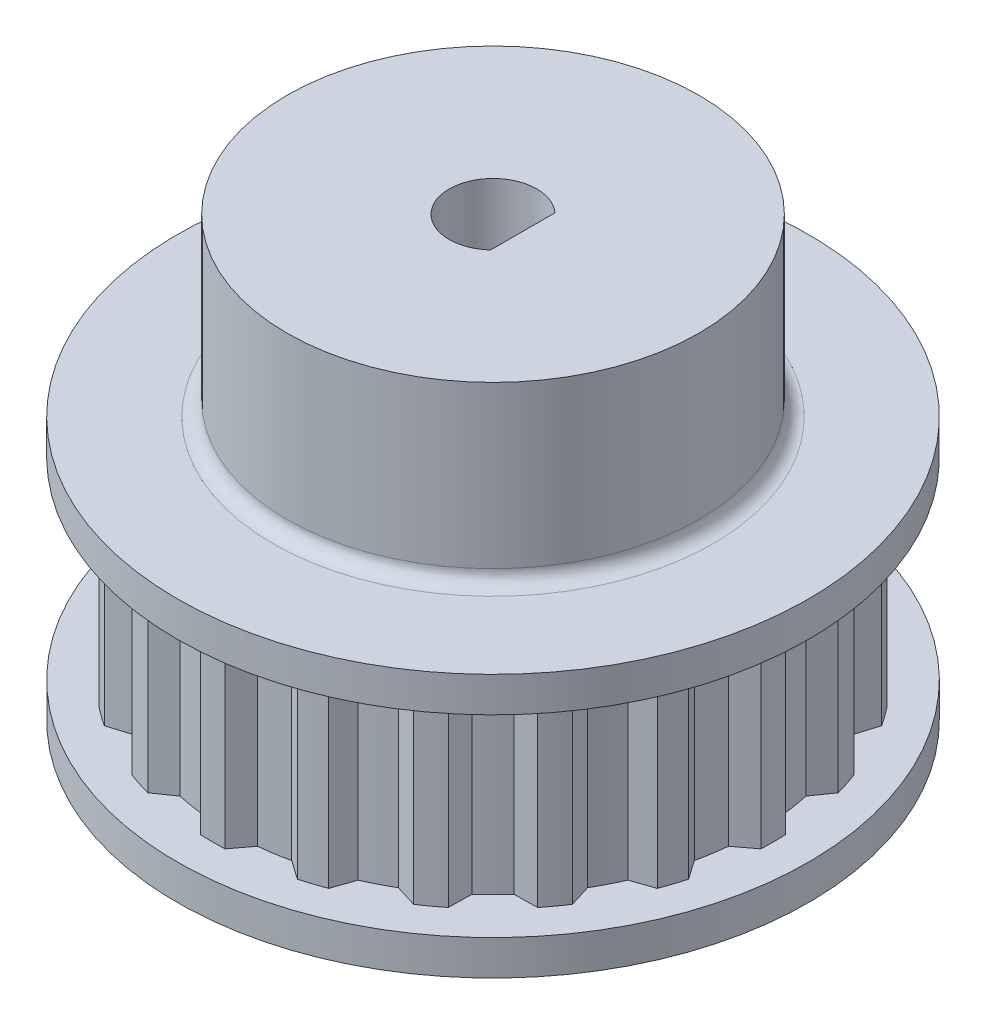
SolidWorks part; units mm, degrees
ref_plane "Front Plane" through (0, 0, 0) normal (0, 0, 1) x (1, 0, 0)
ref_plane "Top Plane" through (0, 0, 0) normal (0, 1, 0) x (1, 0, 0)
ref_plane "Right Plane" through (0, 0, 0) normal (1, 0, 0) x (0, 0, -1)
sketch "Sketch1" plane through (0, 0, 0) normal (0, 1, 0) x (1, 0, 0)
  circle A0 centre (0, 0) radius 16
  dimension "D1" = 32
extrude "Boss-Extrude1" add sketch "Sketch1" along normal blind 11
sketch "Sketch2" plane through (0, 11, 0) normal (0, 1, 0) x (1, 0, 0)
  line L0 (0, 21.2272) -> (0, -27.4763) construction
  line L1 (-1.5, 14.9329) -> (-0.7089, 15.9843)
  line L2 (1.5, 14.9329) -> (0.7089, 15.9843)
  line L3 (3.1879, 14.6656) -> (4.2652, 15.421)
  line L4 (6.0411, 13.7385) -> (5.6137, 14.9829)
  line L5 (7.5638, 12.9627) -> (8.8218, 13.3483)
  line L6 (9.9909, 11.1993) -> (9.9689, 12.5149)
  line L7 (11.1993, 9.9909) -> (12.5149, 9.9689)
  line L8 (12.9627, 7.5638) -> (13.3483, 8.8218)
  line L9 (13.7385, 6.0411) -> (14.9829, 5.6137)
  line L10 (14.6656, 3.1879) -> (15.421, 4.2652)
  line L11 (14.9329, 1.5) -> (15.9843, 0.7089)
  line L12 (14.9329, -1.5) -> (15.9843, -0.7089)
  line L13 (14.6656, -3.1879) -> (15.421, -4.2652)
  line L14 (13.7385, -6.0411) -> (14.9829, -5.6137)
  line L15 (12.9627, -7.5638) -> (13.3483, -8.8218)
  line L16 (11.1993, -9.9909) -> (12.5149, -9.9689)
  line L17 (9.9909, -11.1993) -> (9.9689, -12.5149)
  line L18 (7.5638, -12.9627) -> (8.8218, -13.3483)
  line L19 (6.0411, -13.7385) -> (5.6137, -14.9829)
  line L20 (3.1879, -14.6656) -> (4.2652, -15.421)
  line L21 (1.5, -14.9329) -> (0.7089, -15.9843)
  line L22 (-1.5, -14.9329) -> (-0.7089, -15.9843)
  line L23 (-3.1879, -14.6656) -> (-4.2652, -15.421)
  line L24 (-6.0411, -13.7385) -> (-5.6137, -14.9829)
  line L25 (-7.5638, -12.9627) -> (-8.8218, -13.3483)
  line L26 (-9.9909, -11.1993) -> (-9.9689, -12.5149)
  line L27 (-11.1993, -9.9909) -> (-12.5149, -9.9689)
  line L28 (-12.9627, -7.5638) -> (-13.3483, -8.8218)
  line L29 (-13.7385, -6.0411) -> (-14.9829, -5.6137)
  line L30 (-14.6656, -3.1879) -> (-15.421, -4.2652)
  line L31 (-14.9329, -1.5) -> (-15.9843, -0.7089)
  line L32 (-14.9329, 1.5) -> (-15.9843, 0.7089)
  line L33 (-14.6656, 3.1879) -> (-15.421, 4.2652)
  line L34 (-13.7385, 6.0411) -> (-14.9829, 5.6137)
  line L35 (-12.9627, 7.5638) -> (-13.3483, 8.8218)
  line L36 (-11.1993, 9.9909) -> (-12.5149, 9.9689)
  line L37 (-9.9909, 11.1993) -> (-9.9689, 12.5149)
  line L38 (-7.5638, 12.9627) -> (-8.8218, 13.3483)
  line L39 (-6.0411, 13.7385) -> (-5.6137, 14.9829)
  line L40 (-3.1879, 14.6656) -> (-4.2652, 15.421)
  arc A0 (-1.5, 14.9329) -> (-3.1879, 14.6656) centre (0, 0) ccw
  circle A1 centre (0, 0) radius 16 construction
  arc A3 (-1.5, 14.9329) -> (-3.1879, 14.6656) centre (0, 0) ccw
  arc A4 (5.6137, 14.9829) -> (4.2652, 15.421) centre (0, 0) ccw
  arc A5 (-1.5, 14.9329) -> (-3.1879, 14.6656) centre (0, 0) ccw
  arc A6 (9.9689, 12.5149) -> (8.8218, 13.3483) centre (0, 0) ccw
  arc A7 (-1.5, 14.9329) -> (-3.1879, 14.6656) centre (0, 0) ccw
  arc A8 (13.3483, 8.8218) -> (12.5149, 9.9689) centre (0, 0) ccw
  arc A9 (-1.5, 14.9329) -> (-3.1879, 14.6656) centre (0, 0) ccw
  arc A10 (15.9843, 0.7089) -> (15.421, 4.2652) centre (0, 0) ccw
  arc A11 (-1.5, 14.9329) -> (-3.1879, 14.6656) centre (0, 0) ccw
  arc A12 (15.421, -4.2652) -> (15.9843, -0.7089) centre (0, 0) ccw
  arc A13 (-1.5, 14.9329) -> (-3.1879, 14.6656) centre (0, 0) ccw
  arc A14 (13.3483, -8.8218) -> (14.9829, -5.6137) centre (0, 0) ccw
  arc A15 (-1.5, 14.9329) -> (-3.1879, 14.6656) centre (0, 0) ccw
  arc A16 (9.9689, -12.5149) -> (12.5149, -9.9689) centre (0, 0) ccw
  arc A17 (-1.5, 14.9329) -> (-3.1879, 14.6656) centre (0, 0) ccw
  arc A18 (5.6137, -14.9829) -> (8.8218, -13.3483) centre (0, 0) ccw
  arc A19 (-1.5, 14.9329) -> (-3.1879, 14.6656) centre (0, 0) ccw
  arc A20 (0.7089, -15.9843) -> (4.2652, -15.421) centre (0, 0) ccw
  arc A21 (-1.5, 14.9329) -> (-3.1879, 14.6656) centre (0, 0) ccw
  arc A22 (-4.2652, -15.421) -> (-0.7089, -15.9843) centre (0, 0) ccw
  arc A23 (-1.5, 14.9329) -> (-3.1879, 14.6656) centre (0, 0) ccw
  arc A24 (-8.8218, -13.3483) -> (-5.6137, -14.9829) centre (0, 0) ccw
  arc A25 (-1.5, 14.9329) -> (-3.1879, 14.6656) centre (0, 0) ccw
  arc A26 (-12.5149, -9.9689) -> (-9.9689, -12.5149) centre (0, 0) ccw
  arc A27 (-1.5, 14.9329) -> (-3.1879, 14.6656) centre (0, 0) ccw
  arc A28 (-14.9829, -5.6137) -> (-13.3483, -8.8218) centre (0, 0) ccw
  arc A29 (-1.5, 14.9329) -> (-3.1879, 14.6656) centre (0, 0) ccw
  arc A30 (-15.9843, -0.7089) -> (-15.421, -4.2652) centre (0, 0) ccw
  arc A31 (-1.5, 14.9329) -> (-3.1879, 14.6656) centre (0, 0) ccw
  arc A32 (-15.421, 4.2652) -> (-15.9843, 0.7089) centre (0, 0) ccw
  arc A33 (-1.5, 14.9329) -> (-3.1879, 14.6656) centre (0, 0) ccw
  arc A34 (-13.3483, 8.8218) -> (-14.9829, 5.6137) centre (0, 0) ccw
  arc A35 (-1.5, 14.9329) -> (-3.1879, 14.6656) centre (0, 0) ccw
  arc A36 (-9.9689, 12.5149) -> (-12.5149, 9.9689) centre (0, 0) ccw
  arc A37 (-1.5, 14.9329) -> (-3.1879, 14.6656) centre (0, 0) ccw
  arc A38 (-5.6137, 14.9829) -> (-8.8218, 13.3483) centre (0, 0) ccw
  arc A39 (-1.5, 14.9329) -> (-3.1879, 14.6656) centre (0, 0) ccw
  arc A40 (-0.7089, 15.9843) -> (-4.2652, 15.421) centre (0, 0) ccw
  arc A41 (3.1879, 14.6656) -> (1.5, 14.9329) centre (0, 0) ccw
  arc A42 (3.1879, 14.6656) -> (1.5, 14.9329) centre (0, 0) ccw
  arc A43 (3.1879, 14.6656) -> (1.5, 14.9329) centre (0, 0) ccw
  arc A44 (3.1879, 14.6656) -> (1.5, 14.9329) centre (0, 0) ccw
  arc A45 (3.1879, 14.6656) -> (1.5, 14.9329) centre (0, 0) ccw
  arc A46 (3.1879, 14.6656) -> (1.5, 14.9329) centre (0, 0) ccw
  arc A47 (3.1879, 14.6656) -> (1.5, 14.9329) centre (0, 0) ccw
  arc A48 (3.1879, 14.6656) -> (1.5, 14.9329) centre (0, 0) ccw
  arc A49 (3.1879, 14.6656) -> (1.5, 14.9329) centre (0, 0) ccw
  arc A50 (3.1879, 14.6656) -> (1.5, 14.9329) centre (0, 0) ccw
  arc A51 (3.1879, 14.6656) -> (1.5, 14.9329) centre (0, 0) ccw
  arc A52 (3.1879, 14.6656) -> (1.5, 14.9329) centre (0, 0) ccw
  arc A53 (3.1879, 14.6656) -> (1.5, 14.9329) centre (0, 0) ccw
  arc A54 (3.1879, 14.6656) -> (1.5, 14.9329) centre (0, 0) ccw
  arc A55 (3.1879, 14.6656) -> (1.5, 14.9329) centre (0, 0) ccw
  arc A56 (3.1879, 14.6656) -> (1.5, 14.9329) centre (0, 0) ccw
  arc A57 (3.1879, 14.6656) -> (1.5, 14.9329) centre (0, 0) ccw
  arc A58 (3.1879, 14.6656) -> (1.5, 14.9329) centre (0, 0) ccw
  arc A59 (3.1879, 14.6656) -> (1.5, 14.9329) centre (0, 0) ccw
  arc A60 (3.1879, 14.6656) -> (1.5, 14.9329) centre (0, 0) ccw
  arc A61 (7.5638, 12.9627) -> (6.0411, 13.7385) centre (0, 0) ccw
  arc A62 (7.5638, 12.9627) -> (6.0411, 13.7385) centre (0, 0) ccw
  arc A63 (7.5638, 12.9627) -> (6.0411, 13.7385) centre (0, 0) ccw
  arc A64 (7.5638, 12.9627) -> (6.0411, 13.7385) centre (0, 0) ccw
  arc A65 (7.5638, 12.9627) -> (6.0411, 13.7385) centre (0, 0) ccw
  arc A66 (7.5638, 12.9627) -> (6.0411, 13.7385) centre (0, 0) ccw
  arc A67 (7.5638, 12.9627) -> (6.0411, 13.7385) centre (0, 0) ccw
  arc A68 (7.5638, 12.9627) -> (6.0411, 13.7385) centre (0, 0) ccw
  arc A69 (7.5638, 12.9627) -> (6.0411, 13.7385) centre (0, 0) ccw
  arc A70 (7.5638, 12.9627) -> (6.0411, 13.7385) centre (0, 0) ccw
  arc A71 (7.5638, 12.9627) -> (6.0411, 13.7385) centre (0, 0) ccw
  arc A72 (7.5638, 12.9627) -> (6.0411, 13.7385) centre (0, 0) ccw
  arc A73 (7.5638, 12.9627) -> (6.0411, 13.7385) centre (0, 0) ccw
  arc A74 (7.5638, 12.9627) -> (6.0411, 13.7385) centre (0, 0) ccw
  arc A75 (7.5638, 12.9627) -> (6.0411, 13.7385) centre (0, 0) ccw
  arc A76 (7.5638, 12.9627) -> (6.0411, 13.7385) centre (0, 0) ccw
  arc A77 (7.5638, 12.9627) -> (6.0411, 13.7385) centre (0, 0) ccw
  arc A78 (7.5638, 12.9627) -> (6.0411, 13.7385) centre (0, 0) ccw
  arc A79 (7.5638, 12.9627) -> (6.0411, 13.7385) centre (0, 0) ccw
  arc A80 (7.5638, 12.9627) -> (6.0411, 13.7385) centre (0, 0) ccw
  arc A81 (11.1993, 9.9909) -> (9.9909, 11.1993) centre (0, 0) ccw
  arc A82 (11.1993, 9.9909) -> (9.9909, 11.1993) centre (0, 0) ccw
  arc A83 (11.1993, 9.9909) -> (9.9909, 11.1993) centre (0, 0) ccw
  arc A84 (11.1993, 9.9909) -> (9.9909, 11.1993) centre (0, 0) ccw
  arc A85 (11.1993, 9.9909) -> (9.9909, 11.1993) centre (0, 0) ccw
  arc A86 (11.1993, 9.9909) -> (9.9909, 11.1993) centre (0, 0) ccw
  arc A87 (11.1993, 9.9909) -> (9.9909, 11.1993) centre (0, 0) ccw
  arc A88 (11.1993, 9.9909) -> (9.9909, 11.1993) centre (0, 0) ccw
  arc A89 (11.1993, 9.9909) -> (9.9909, 11.1993) centre (0, 0) ccw
  arc A90 (11.1993, 9.9909) -> (9.9909, 11.1993) centre (0, 0) ccw
  arc A91 (11.1993, 9.9909) -> (9.9909, 11.1993) centre (0, 0) ccw
  arc A92 (11.1993, 9.9909) -> (9.9909, 11.1993) centre (0, 0) ccw
  arc A93 (11.1993, 9.9909) -> (9.9909, 11.1993) centre (0, 0) ccw
  arc A94 (11.1993, 9.9909) -> (9.9909, 11.1993) centre (0, 0) ccw
  arc A95 (11.1993, 9.9909) -> (9.9909, 11.1993) centre (0, 0) ccw
  arc A96 (11.1993, 9.9909) -> (9.9909, 11.1993) centre (0, 0) ccw
  arc A97 (11.1993, 9.9909) -> (9.9909, 11.1993) centre (0, 0) ccw
  arc A98 (11.1993, 9.9909) -> (9.9909, 11.1993) centre (0, 0) ccw
  arc A99 (11.1993, 9.9909) -> (9.9909, 11.1993) centre (0, 0) ccw
  arc A100 (11.1993, 9.9909) -> (9.9909, 11.1993) centre (0, 0) ccw
  arc A101 (13.7385, 6.0411) -> (12.9627, 7.5638) centre (0, 0) ccw
  arc A102 (13.7385, 6.0411) -> (12.9627, 7.5638) centre (0, 0) ccw
  arc A103 (13.7385, 6.0411) -> (12.9627, 7.5638) centre (0, 0) ccw
  arc A104 (13.7385, 6.0411) -> (12.9627, 7.5638) centre (0, 0) ccw
  arc A105 (13.7385, 6.0411) -> (12.9627, 7.5638) centre (0, 0) ccw
  arc A106 (13.7385, 6.0411) -> (12.9627, 7.5638) centre (0, 0) ccw
  arc A107 (13.7385, 6.0411) -> (12.9627, 7.5638) centre (0, 0) ccw
  arc A108 (13.7385, 6.0411) -> (12.9627, 7.5638) centre (0, 0) ccw
  arc A109 (13.7385, 6.0411) -> (12.9627, 7.5638) centre (0, 0) ccw
  arc A110 (13.7385, 6.0411) -> (12.9627, 7.5638) centre (0, 0) ccw
  arc A111 (13.7385, 6.0411) -> (12.9627, 7.5638) centre (0, 0) ccw
  arc A112 (13.7385, 6.0411) -> (12.9627, 7.5638) centre (0, 0) ccw
  arc A113 (13.7385, 6.0411) -> (12.9627, 7.5638) centre (0, 0) ccw
  arc A114 (13.7385, 6.0411) -> (12.9627, 7.5638) centre (0, 0) ccw
  arc A115 (13.7385, 6.0411) -> (12.9627, 7.5638) centre (0, 0) ccw
  arc A116 (13.7385, 6.0411) -> (12.9627, 7.5638) centre (0, 0) ccw
  arc A117 (13.7385, 6.0411) -> (12.9627, 7.5638) centre (0, 0) ccw
  arc A118 (13.7385, 6.0411) -> (12.9627, 7.5638) centre (0, 0) ccw
  arc A119 (13.7385, 6.0411) -> (12.9627, 7.5638) centre (0, 0) ccw
  arc A120 (13.7385, 6.0411) -> (12.9627, 7.5638) centre (0, 0) ccw
  arc A121 (14.9329, 1.5) -> (14.6656, 3.1879) centre (0, 0) ccw
  arc A122 (14.9329, 1.5) -> (14.6656, 3.1879) centre (0, 0) ccw
  arc A123 (14.9329, 1.5) -> (14.6656, 3.1879) centre (0, 0) ccw
  arc A124 (14.9329, 1.5) -> (14.6656, 3.1879) centre (0, 0) ccw
  arc A125 (14.9329, 1.5) -> (14.6656, 3.1879) centre (0, 0) ccw
  arc A126 (14.9329, 1.5) -> (14.6656, 3.1879) centre (0, 0) ccw
  arc A127 (14.9329, 1.5) -> (14.6656, 3.1879) centre (0, 0) ccw
  arc A128 (14.9329, 1.5) -> (14.6656, 3.1879) centre (0, 0) ccw
  arc A129 (14.9329, 1.5) -> (14.6656, 3.1879) centre (0, 0) ccw
  arc A130 (14.9329, 1.5) -> (14.6656, 3.1879) centre (0, 0) ccw
  arc A131 (14.9329, 1.5) -> (14.6656, 3.1879) centre (0, 0) ccw
  arc A132 (14.9329, 1.5) -> (14.6656, 3.1879) centre (0, 0) ccw
  arc A133 (14.9329, 1.5) -> (14.6656, 3.1879) centre (0, 0) ccw
  arc A134 (14.9329, 1.5) -> (14.6656, 3.1879) centre (0, 0) ccw
  arc A135 (14.9329, 1.5) -> (14.6656, 3.1879) centre (0, 0) ccw
  arc A136 (14.9329, 1.5) -> (14.6656, 3.1879) centre (0, 0) ccw
  arc A137 (14.9329, 1.5) -> (14.6656, 3.1879) centre (0, 0) ccw
  arc A138 (14.9329, 1.5) -> (14.6656, 3.1879) centre (0, 0) ccw
  arc A139 (14.9329, 1.5) -> (14.6656, 3.1879) centre (0, 0) ccw
  arc A140 (14.9329, 1.5) -> (14.6656, 3.1879) centre (0, 0) ccw
  arc A141 (14.6656, -3.1879) -> (14.9329, -1.5) centre (0, 0) ccw
  arc A142 (14.6656, -3.1879) -> (14.9329, -1.5) centre (0, 0) ccw
  arc A143 (14.6656, -3.1879) -> (14.9329, -1.5) centre (0, 0) ccw
  arc A144 (14.6656, -3.1879) -> (14.9329, -1.5) centre (0, 0) ccw
  arc A145 (14.6656, -3.1879) -> (14.9329, -1.5) centre (0, 0) ccw
  arc A146 (14.6656, -3.1879) -> (14.9329, -1.5) centre (0, 0) ccw
  arc A147 (14.6656, -3.1879) -> (14.9329, -1.5) centre (0, 0) ccw
  arc A148 (14.6656, -3.1879) -> (14.9329, -1.5) centre (0, 0) ccw
  arc A149 (14.6656, -3.1879) -> (14.9329, -1.5) centre (0, 0) ccw
  arc A150 (14.6656, -3.1879) -> (14.9329, -1.5) centre (0, 0) ccw
  arc A151 (14.6656, -3.1879) -> (14.9329, -1.5) centre (0, 0) ccw
  arc A152 (14.6656, -3.1879) -> (14.9329, -1.5) centre (0, 0) ccw
  arc A153 (14.6656, -3.1879) -> (14.9329, -1.5) centre (0, 0) ccw
  arc A154 (14.6656, -3.1879) -> (14.9329, -1.5) centre (0, 0) ccw
  arc A155 (14.6656, -3.1879) -> (14.9329, -1.5) centre (0, 0) ccw
  arc A156 (14.6656, -3.1879) -> (14.9329, -1.5) centre (0, 0) ccw
  arc A157 (14.6656, -3.1879) -> (14.9329, -1.5) centre (0, 0) ccw
  arc A158 (14.6656, -3.1879) -> (14.9329, -1.5) centre (0, 0) ccw
  arc A159 (14.6656, -3.1879) -> (14.9329, -1.5) centre (0, 0) ccw
  arc A160 (14.6656, -3.1879) -> (14.9329, -1.5) centre (0, 0) ccw
  arc A161 (12.9627, -7.5638) -> (13.7385, -6.0411) centre (0, 0) ccw
  arc A162 (12.9627, -7.5638) -> (13.7385, -6.0411) centre (0, 0) ccw
  arc A163 (12.9627, -7.5638) -> (13.7385, -6.0411) centre (0, 0) ccw
  arc A164 (12.9627, -7.5638) -> (13.7385, -6.0411) centre (0, 0) ccw
  arc A165 (12.9627, -7.5638) -> (13.7385, -6.0411) centre (0, 0) ccw
  arc A166 (12.9627, -7.5638) -> (13.7385, -6.0411) centre (0, 0) ccw
  arc A167 (12.9627, -7.5638) -> (13.7385, -6.0411) centre (0, 0) ccw
  arc A168 (12.9627, -7.5638) -> (13.7385, -6.0411) centre (0, 0) ccw
  arc A169 (12.9627, -7.5638) -> (13.7385, -6.0411) centre (0, 0) ccw
  arc A170 (12.9627, -7.5638) -> (13.7385, -6.0411) centre (0, 0) ccw
  arc A171 (12.9627, -7.5638) -> (13.7385, -6.0411) centre (0, 0) ccw
  arc A172 (12.9627, -7.5638) -> (13.7385, -6.0411) centre (0, 0) ccw
  arc A173 (12.9627, -7.5638) -> (13.7385, -6.0411) centre (0, 0) ccw
  arc A174 (12.9627, -7.5638) -> (13.7385, -6.0411) centre (0, 0) ccw
  arc A175 (12.9627, -7.5638) -> (13.7385, -6.0411) centre (0, 0) ccw
  arc A176 (12.9627, -7.5638) -> (13.7385, -6.0411) centre (0, 0) ccw
  arc A177 (12.9627, -7.5638) -> (13.7385, -6.0411) centre (0, 0) ccw
  arc A178 (12.9627, -7.5638) -> (13.7385, -6.0411) centre (0, 0) ccw
  arc A179 (12.9627, -7.5638) -> (13.7385, -6.0411) centre (0, 0) ccw
  arc A180 (12.9627, -7.5638) -> (13.7385, -6.0411) centre (0, 0) ccw
  arc A181 (9.9909, -11.1993) -> (11.1993, -9.9909) centre (0, 0) ccw
  arc A182 (9.9909, -11.1993) -> (11.1993, -9.9909) centre (0, 0) ccw
  arc A183 (9.9909, -11.1993) -> (11.1993, -9.9909) centre (0, 0) ccw
  arc A184 (9.9909, -11.1993) -> (11.1993, -9.9909) centre (0, 0) ccw
  arc A185 (9.9909, -11.1993) -> (11.1993, -9.9909) centre (0, 0) ccw
  arc A186 (9.9909, -11.1993) -> (11.1993, -9.9909) centre (0, 0) ccw
  arc A187 (9.9909, -11.1993) -> (11.1993, -9.9909) centre (0, 0) ccw
  arc A188 (9.9909, -11.1993) -> (11.1993, -9.9909) centre (0, 0) ccw
  arc A189 (9.9909, -11.1993) -> (11.1993, -9.9909) centre (0, 0) ccw
  arc A190 (9.9909, -11.1993) -> (11.1993, -9.9909) centre (0, 0) ccw
  arc A191 (9.9909, -11.1993) -> (11.1993, -9.9909) centre (0, 0) ccw
  arc A192 (9.9909, -11.1993) -> (11.1993, -9.9909) centre (0, 0) ccw
  arc A193 (9.9909, -11.1993) -> (11.1993, -9.9909) centre (0, 0) ccw
  arc A194 (9.9909, -11.1993) -> (11.1993, -9.9909) centre (0, 0) ccw
  arc A195 (9.9909, -11.1993) -> (11.1993, -9.9909) centre (0, 0) ccw
  arc A196 (9.9909, -11.1993) -> (11.1993, -9.9909) centre (0, 0) ccw
  arc A197 (9.9909, -11.1993) -> (11.1993, -9.9909) centre (0, 0) ccw
  arc A198 (9.9909, -11.1993) -> (11.1993, -9.9909) centre (0, 0) ccw
  arc A199 (9.9909, -11.1993) -> (11.1993, -9.9909) centre (0, 0) ccw
  arc A200 (9.9909, -11.1993) -> (11.1993, -9.9909) centre (0, 0) ccw
  arc A201 (1.5, -14.9329) -> (3.1879, -14.6656) centre (0, 0) ccw
  arc A202 (1.5, -14.9329) -> (3.1879, -14.6656) centre (0, 0) ccw
  arc A203 (1.5, -14.9329) -> (3.1879, -14.6656) centre (0, 0) ccw
  arc A204 (1.5, -14.9329) -> (3.1879, -14.6656) centre (0, 0) ccw
  arc A205 (1.5, -14.9329) -> (3.1879, -14.6656) centre (0, 0) ccw
  arc A206 (1.5, -14.9329) -> (3.1879, -14.6656) centre (0, 0) ccw
  arc A207 (1.5, -14.9329) -> (3.1879, -14.6656) centre (0, 0) ccw
  arc A208 (1.5, -14.9329) -> (3.1879, -14.6656) centre (0, 0) ccw
  arc A209 (1.5, -14.9329) -> (3.1879, -14.6656) centre (0, 0) ccw
  arc A210 (1.5, -14.9329) -> (3.1879, -14.6656) centre (0, 0) ccw
  arc A211 (1.5, -14.9329) -> (3.1879, -14.6656) centre (0, 0) ccw
  arc A212 (1.5, -14.9329) -> (3.1879, -14.6656) centre (0, 0) ccw
  arc A213 (1.5, -14.9329) -> (3.1879, -14.6656) centre (0, 0) ccw
  arc A214 (1.5, -14.9329) -> (3.1879, -14.6656) centre (0, 0) ccw
  arc A215 (1.5, -14.9329) -> (3.1879, -14.6656) centre (0, 0) ccw
  arc A216 (1.5, -14.9329) -> (3.1879, -14.6656) centre (0, 0) ccw
  arc A217 (1.5, -14.9329) -> (3.1879, -14.6656) centre (0, 0) ccw
  arc A218 (1.5, -14.9329) -> (3.1879, -14.6656) centre (0, 0) ccw
  arc A219 (1.5, -14.9329) -> (3.1879, -14.6656) centre (0, 0) ccw
  arc A220 (1.5, -14.9329) -> (3.1879, -14.6656) centre (0, 0) ccw
  arc A221 (-3.1879, -14.6656) -> (-1.5, -14.9329) centre (0, 0) ccw
  arc A222 (-3.1879, -14.6656) -> (-1.5, -14.9329) centre (0, 0) ccw
  arc A223 (-3.1879, -14.6656) -> (-1.5, -14.9329) centre (0, 0) ccw
  arc A224 (-3.1879, -14.6656) -> (-1.5, -14.9329) centre (0, 0) ccw
  arc A225 (-3.1879, -14.6656) -> (-1.5, -14.9329) centre (0, 0) ccw
  arc A226 (-3.1879, -14.6656) -> (-1.5, -14.9329) centre (0, 0) ccw
  arc A227 (-3.1879, -14.6656) -> (-1.5, -14.9329) centre (0, 0) ccw
  arc A228 (-3.1879, -14.6656) -> (-1.5, -14.9329) centre (0, 0) ccw
  arc A229 (-3.1879, -14.6656) -> (-1.5, -14.9329) centre (0, 0) ccw
  arc A230 (-3.1879, -14.6656) -> (-1.5, -14.9329) centre (0, 0) ccw
  arc A231 (-3.1879, -14.6656) -> (-1.5, -14.9329) centre (0, 0) ccw
  arc A232 (-3.1879, -14.6656) -> (-1.5, -14.9329) centre (0, 0) ccw
  arc A233 (-3.1879, -14.6656) -> (-1.5, -14.9329) centre (0, 0) ccw
  arc A234 (-3.1879, -14.6656) -> (-1.5, -14.9329) centre (0, 0) ccw
  arc A235 (-3.1879, -14.6656) -> (-1.5, -14.9329) centre (0, 0) ccw
  arc A236 (-3.1879, -14.6656) -> (-1.5, -14.9329) centre (0, 0) ccw
  arc A237 (-3.1879, -14.6656) -> (-1.5, -14.9329) centre (0, 0) ccw
  arc A238 (-3.1879, -14.6656) -> (-1.5, -14.9329) centre (0, 0) ccw
  arc A239 (-3.1879, -14.6656) -> (-1.5, -14.9329) centre (0, 0) ccw
  arc A240 (-3.1879, -14.6656) -> (-1.5, -14.9329) centre (0, 0) ccw
  arc A241 (-7.5638, -12.9627) -> (-6.0411, -13.7385) centre (0, 0) ccw
  arc A242 (-7.5638, -12.9627) -> (-6.0411, -13.7385) centre (0, 0) ccw
  arc A243 (-7.5638, -12.9627) -> (-6.0411, -13.7385) centre (0, 0) ccw
  arc A244 (-7.5638, -12.9627) -> (-6.0411, -13.7385) centre (0, 0) ccw
  arc A245 (-7.5638, -12.9627) -> (-6.0411, -13.7385) centre (0, 0) ccw
  arc A246 (-7.5638, -12.9627) -> (-6.0411, -13.7385) centre (0, 0) ccw
  arc A247 (-7.5638, -12.9627) -> (-6.0411, -13.7385) centre (0, 0) ccw
  arc A248 (-7.5638, -12.9627) -> (-6.0411, -13.7385) centre (0, 0) ccw
  arc A249 (-7.5638, -12.9627) -> (-6.0411, -13.7385) centre (0, 0) ccw
  arc A250 (-7.5638, -12.9627) -> (-6.0411, -13.7385) centre (0, 0) ccw
  arc A251 (-7.5638, -12.9627) -> (-6.0411, -13.7385) centre (0, 0) ccw
  arc A252 (-7.5638, -12.9627) -> (-6.0411, -13.7385) centre (0, 0) ccw
  arc A253 (-7.5638, -12.9627) -> (-6.0411, -13.7385) centre (0, 0) ccw
  arc A254 (-7.5638, -12.9627) -> (-6.0411, -13.7385) centre (0, 0) ccw
  arc A255 (-7.5638, -12.9627) -> (-6.0411, -13.7385) centre (0, 0) ccw
  arc A256 (-7.5638, -12.9627) -> (-6.0411, -13.7385) centre (0, 0) ccw
  arc A257 (-7.5638, -12.9627) -> (-6.0411, -13.7385) centre (0, 0) ccw
  arc A258 (-7.5638, -12.9627) -> (-6.0411, -13.7385) centre (0, 0) ccw
  arc A259 (-7.5638, -12.9627) -> (-6.0411, -13.7385) centre (0, 0) ccw
  arc A260 (-7.5638, -12.9627) -> (-6.0411, -13.7385) centre (0, 0) ccw
  arc A261 (-11.1993, -9.9909) -> (-9.9909, -11.1993) centre (0, 0) ccw
  arc A262 (-11.1993, -9.9909) -> (-9.9909, -11.1993) centre (0, 0) ccw
  arc A263 (-11.1993, -9.9909) -> (-9.9909, -11.1993) centre (0, 0) ccw
  arc A264 (-11.1993, -9.9909) -> (-9.9909, -11.1993) centre (0, 0) ccw
  arc A265 (-11.1993, -9.9909) -> (-9.9909, -11.1993) centre (0, 0) ccw
  arc A266 (-11.1993, -9.9909) -> (-9.9909, -11.1993) centre (0, 0) ccw
  arc A267 (-11.1993, -9.9909) -> (-9.9909, -11.1993) centre (0, 0) ccw
  arc A268 (-11.1993, -9.9909) -> (-9.9909, -11.1993) centre (0, 0) ccw
  arc A269 (-11.1993, -9.9909) -> (-9.9909, -11.1993) centre (0, 0) ccw
  arc A270 (-11.1993, -9.9909) -> (-9.9909, -11.1993) centre (0, 0) ccw
  arc A271 (-11.1993, -9.9909) -> (-9.9909, -11.1993) centre (0, 0) ccw
  arc A272 (-11.1993, -9.9909) -> (-9.9909, -11.1993) centre (0, 0) ccw
  arc A273 (-11.1993, -9.9909) -> (-9.9909, -11.1993) centre (0, 0) ccw
  arc A274 (-11.1993, -9.9909) -> (-9.9909, -11.1993) centre (0, 0) ccw
  arc A275 (-11.1993, -9.9909) -> (-9.9909, -11.1993) centre (0, 0) ccw
  arc A276 (-11.1993, -9.9909) -> (-9.9909, -11.1993) centre (0, 0) ccw
  arc A277 (-11.1993, -9.9909) -> (-9.9909, -11.1993) centre (0, 0) ccw
  arc A278 (-11.1993, -9.9909) -> (-9.9909, -11.1993) centre (0, 0) ccw
  arc A279 (-11.1993, -9.9909) -> (-9.9909, -11.1993) centre (0, 0) ccw
  arc A280 (-11.1993, -9.9909) -> (-9.9909, -11.1993) centre (0, 0) ccw
  arc A281 (-13.7385, -6.0411) -> (-12.9627, -7.5638) centre (0, 0) ccw
  arc A282 (-13.7385, -6.0411) -> (-12.9627, -7.5638) centre (0, 0) ccw
  arc A283 (-13.7385, -6.0411) -> (-12.9627, -7.5638) centre (0, 0) ccw
  arc A284 (-13.7385, -6.0411) -> (-12.9627, -7.5638) centre (0, 0) ccw
  arc A285 (-13.7385, -6.0411) -> (-12.9627, -7.5638) centre (0, 0) ccw
  arc A286 (-13.7385, -6.0411) -> (-12.9627, -7.5638) centre (0, 0) ccw
  arc A287 (-13.7385, -6.0411) -> (-12.9627, -7.5638) centre (0, 0) ccw
  arc A288 (-13.7385, -6.0411) -> (-12.9627, -7.5638) centre (0, 0) ccw
  arc A289 (-13.7385, -6.0411) -> (-12.9627, -7.5638) centre (0, 0) ccw
  arc A290 (-13.7385, -6.0411) -> (-12.9627, -7.5638) centre (0, 0) ccw
  arc A291 (-13.7385, -6.0411) -> (-12.9627, -7.5638) centre (0, 0) ccw
  arc A292 (-13.7385, -6.0411) -> (-12.9627, -7.5638) centre (0, 0) ccw
  arc A293 (-13.7385, -6.0411) -> (-12.9627, -7.5638) centre (0, 0) ccw
  arc A294 (-13.7385, -6.0411) -> (-12.9627, -7.5638) centre (0, 0) ccw
  arc A295 (-13.7385, -6.0411) -> (-12.9627, -7.5638) centre (0, 0) ccw
  arc A296 (-13.7385, -6.0411) -> (-12.9627, -7.5638) centre (0, 0) ccw
  arc A297 (-13.7385, -6.0411) -> (-12.9627, -7.5638) centre (0, 0) ccw
  arc A298 (-13.7385, -6.0411) -> (-12.9627, -7.5638) centre (0, 0) ccw
  arc A299 (-13.7385, -6.0411) -> (-12.9627, -7.5638) centre (0, 0) ccw
  arc A300 (-13.7385, -6.0411) -> (-12.9627, -7.5638) centre (0, 0) ccw
  arc A301 (-14.9329, -1.5) -> (-14.6656, -3.1879) centre (0, 0) ccw
  arc A302 (-14.9329, -1.5) -> (-14.6656, -3.1879) centre (0, 0) ccw
  arc A303 (-14.9329, -1.5) -> (-14.6656, -3.1879) centre (0, 0) ccw
  arc A304 (-14.9329, -1.5) -> (-14.6656, -3.1879) centre (0, 0) ccw
  arc A305 (-14.9329, -1.5) -> (-14.6656, -3.1879) centre (0, 0) ccw
  arc A306 (-14.9329, -1.5) -> (-14.6656, -3.1879) centre (0, 0) ccw
  arc A307 (-14.9329, -1.5) -> (-14.6656, -3.1879) centre (0, 0) ccw
  arc A308 (-14.9329, -1.5) -> (-14.6656, -3.1879) centre (0, 0) ccw
  arc A309 (-14.9329, -1.5) -> (-14.6656, -3.1879) centre (0, 0) ccw
  arc A310 (-14.9329, -1.5) -> (-14.6656, -3.1879) centre (0, 0) ccw
  arc A311 (-14.9329, -1.5) -> (-14.6656, -3.1879) centre (0, 0) ccw
  arc A312 (-14.9329, -1.5) -> (-14.6656, -3.1879) centre (0, 0) ccw
  arc A313 (-14.9329, -1.5) -> (-14.6656, -3.1879) centre (0, 0) ccw
  arc A314 (-14.9329, -1.5) -> (-14.6656, -3.1879) centre (0, 0) ccw
  arc A315 (-14.9329, -1.5) -> (-14.6656, -3.1879) centre (0, 0) ccw
  arc A316 (-14.9329, -1.5) -> (-14.6656, -3.1879) centre (0, 0) ccw
  arc A317 (-14.9329, -1.5) -> (-14.6656, -3.1879) centre (0, 0) ccw
  arc A318 (-14.9329, -1.5) -> (-14.6656, -3.1879) centre (0, 0) ccw
  arc A319 (-14.9329, -1.5) -> (-14.6656, -3.1879) centre (0, 0) ccw
  arc A320 (-14.9329, -1.5) -> (-14.6656, -3.1879) centre (0, 0) ccw
  arc A321 (-14.6656, 3.1879) -> (-14.9329, 1.5) centre (0, 0) ccw
  arc A322 (-14.6656, 3.1879) -> (-14.9329, 1.5) centre (0, 0) ccw
  arc A323 (-14.6656, 3.1879) -> (-14.9329, 1.5) centre (0, 0) ccw
  arc A324 (-14.6656, 3.1879) -> (-14.9329, 1.5) centre (0, 0) ccw
  arc A325 (-14.6656, 3.1879) -> (-14.9329, 1.5) centre (0, 0) ccw
  arc A326 (-14.6656, 3.1879) -> (-14.9329, 1.5) centre (0, 0) ccw
  arc A327 (-14.6656, 3.1879) -> (-14.9329, 1.5) centre (0, 0) ccw
  arc A328 (-14.6656, 3.1879) -> (-14.9329, 1.5) centre (0, 0) ccw
  arc A329 (-14.6656, 3.1879) -> (-14.9329, 1.5) centre (0, 0) ccw
  arc A330 (-14.6656, 3.1879) -> (-14.9329, 1.5) centre (0, 0) ccw
  arc A331 (-14.6656, 3.1879) -> (-14.9329, 1.5) centre (0, 0) ccw
  arc A332 (-14.6656, 3.1879) -> (-14.9329, 1.5) centre (0, 0) ccw
  arc A333 (-14.6656, 3.1879) -> (-14.9329, 1.5) centre (0, 0) ccw
  arc A334 (-14.6656, 3.1879) -> (-14.9329, 1.5) centre (0, 0) ccw
  arc A335 (-14.6656, 3.1879) -> (-14.9329, 1.5) centre (0, 0) ccw
  arc A336 (-14.6656, 3.1879) -> (-14.9329, 1.5) centre (0, 0) ccw
  arc A337 (-14.6656, 3.1879) -> (-14.9329, 1.5) centre (0, 0) ccw
  arc A338 (-14.6656, 3.1879) -> (-14.9329, 1.5) centre (0, 0) ccw
  arc A339 (-14.6656, 3.1879) -> (-14.9329, 1.5) centre (0, 0) ccw
  arc A340 (-14.6656, 3.1879) -> (-14.9329, 1.5) centre (0, 0) ccw
  arc A341 (-12.9627, 7.5638) -> (-13.7385, 6.0411) centre (0, 0) ccw
  arc A342 (-12.9627, 7.5638) -> (-13.7385, 6.0411) centre (0, 0) ccw
  arc A343 (-12.9627, 7.5638) -> (-13.7385, 6.0411) centre (0, 0) ccw
  arc A344 (-12.9627, 7.5638) -> (-13.7385, 6.0411) centre (0, 0) ccw
  arc A345 (-12.9627, 7.5638) -> (-13.7385, 6.0411) centre (0, 0) ccw
  arc A346 (-12.9627, 7.5638) -> (-13.7385, 6.0411) centre (0, 0) ccw
  arc A347 (-12.9627, 7.5638) -> (-13.7385, 6.0411) centre (0, 0) ccw
  arc A348 (-12.9627, 7.5638) -> (-13.7385, 6.0411) centre (0, 0) ccw
  arc A349 (-12.9627, 7.5638) -> (-13.7385, 6.0411) centre (0, 0) ccw
  arc A350 (-12.9627, 7.5638) -> (-13.7385, 6.0411) centre (0, 0) ccw
  arc A351 (-12.9627, 7.5638) -> (-13.7385, 6.0411) centre (0, 0) ccw
  arc A352 (-12.9627, 7.5638) -> (-13.7385, 6.0411) centre (0, 0) ccw
  arc A353 (-12.9627, 7.5638) -> (-13.7385, 6.0411) centre (0, 0) ccw
  arc A354 (-12.9627, 7.5638) -> (-13.7385, 6.0411) centre (0, 0) ccw
  arc A355 (-12.9627, 7.5638) -> (-13.7385, 6.0411) centre (0, 0) ccw
  arc A356 (-12.9627, 7.5638) -> (-13.7385, 6.0411) centre (0, 0) ccw
  arc A357 (-12.9627, 7.5638) -> (-13.7385, 6.0411) centre (0, 0) ccw
  arc A358 (-12.9627, 7.5638) -> (-13.7385, 6.0411) centre (0, 0) ccw
  arc A359 (-12.9627, 7.5638) -> (-13.7385, 6.0411) centre (0, 0) ccw
  arc A360 (-12.9627, 7.5638) -> (-13.7385, 6.0411) centre (0, 0) ccw
  arc A361 (-9.9909, 11.1993) -> (-11.1993, 9.9909) centre (0, 0) ccw
  arc A362 (-9.9909, 11.1993) -> (-11.1993, 9.9909) centre (0, 0) ccw
  arc A363 (-9.9909, 11.1993) -> (-11.1993, 9.9909) centre (0, 0) ccw
  arc A364 (-9.9909, 11.1993) -> (-11.1993, 9.9909) centre (0, 0) ccw
  arc A365 (-9.9909, 11.1993) -> (-11.1993, 9.9909) centre (0, 0) ccw
  arc A366 (-9.9909, 11.1993) -> (-11.1993, 9.9909) centre (0, 0) ccw
  arc A367 (-9.9909, 11.1993) -> (-11.1993, 9.9909) centre (0, 0) ccw
  arc A368 (-9.9909, 11.1993) -> (-11.1993, 9.9909) centre (0, 0) ccw
  arc A369 (-9.9909, 11.1993) -> (-11.1993, 9.9909) centre (0, 0) ccw
  arc A370 (-9.9909, 11.1993) -> (-11.1993, 9.9909) centre (0, 0) ccw
  arc A371 (-9.9909, 11.1993) -> (-11.1993, 9.9909) centre (0, 0) ccw
  arc A372 (-9.9909, 11.1993) -> (-11.1993, 9.9909) centre (0, 0) ccw
  arc A373 (-9.9909, 11.1993) -> (-11.1993, 9.9909) centre (0, 0) ccw
  arc A374 (-9.9909, 11.1993) -> (-11.1993, 9.9909) centre (0, 0) ccw
  arc A375 (-9.9909, 11.1993) -> (-11.1993, 9.9909) centre (0, 0) ccw
  arc A376 (-9.9909, 11.1993) -> (-11.1993, 9.9909) centre (0, 0) ccw
  arc A377 (-9.9909, 11.1993) -> (-11.1993, 9.9909) centre (0, 0) ccw
  arc A378 (-9.9909, 11.1993) -> (-11.1993, 9.9909) centre (0, 0) ccw
  arc A379 (-9.9909, 11.1993) -> (-11.1993, 9.9909) centre (0, 0) ccw
  arc A380 (-9.9909, 11.1993) -> (-11.1993, 9.9909) centre (0, 0) ccw
  arc A381 (-6.0411, 13.7385) -> (-7.5638, 12.9627) centre (0, 0) ccw
  arc A382 (-6.0411, 13.7385) -> (-7.5638, 12.9627) centre (0, 0) ccw
  arc A383 (-6.0411, 13.7385) -> (-7.5638, 12.9627) centre (0, 0) ccw
  arc A384 (-6.0411, 13.7385) -> (-7.5638, 12.9627) centre (0, 0) ccw
  arc A385 (-6.0411, 13.7385) -> (-7.5638, 12.9627) centre (0, 0) ccw
  arc A386 (-6.0411, 13.7385) -> (-7.5638, 12.9627) centre (0, 0) ccw
  arc A387 (-6.0411, 13.7385) -> (-7.5638, 12.9627) centre (0, 0) ccw
  arc A388 (-6.0411, 13.7385) -> (-7.5638, 12.9627) centre (0, 0) ccw
  arc A389 (-6.0411, 13.7385) -> (-7.5638, 12.9627) centre (0, 0) ccw
  arc A390 (-6.0411, 13.7385) -> (-7.5638, 12.9627) centre (0, 0) ccw
  arc A391 (-6.0411, 13.7385) -> (-7.5638, 12.9627) centre (0, 0) ccw
  arc A392 (-6.0411, 13.7385) -> (-7.5638, 12.9627) centre (0, 0) ccw
  arc A393 (-6.0411, 13.7385) -> (-7.5638, 12.9627) centre (0, 0) ccw
  arc A394 (-6.0411, 13.7385) -> (-7.5638, 12.9627) centre (0, 0) ccw
  arc A395 (-6.0411, 13.7385) -> (-7.5638, 12.9627) centre (0, 0) ccw
  arc A396 (-6.0411, 13.7385) -> (-7.5638, 12.9627) centre (0, 0) ccw
  arc A397 (-6.0411, 13.7385) -> (-7.5638, 12.9627) centre (0, 0) ccw
  arc A398 (-6.0411, 13.7385) -> (-7.5638, 12.9627) centre (0, 0) ccw
  arc A399 (-6.0411, 13.7385) -> (-7.5638, 12.9627) centre (0, 0) ccw
  arc A400 (-6.0411, 13.7385) -> (-7.5638, 12.9627) centre (0, 0) ccw
  arc A401 (14.9829, 5.6137) -> (0.7089, 15.9843) centre (0, 0) ccw
  arc A402 (6.0411, -13.7385) -> (7.5638, -12.9627) centre (0, 0) ccw
  arc A403 (6.0411, -13.7385) -> (7.5638, -12.9627) centre (0, 0) ccw
  arc A404 (6.0411, -13.7385) -> (7.5638, -12.9627) centre (0, 0) ccw
  arc A405 (6.0411, -13.7385) -> (7.5638, -12.9627) centre (0, 0) ccw
  arc A406 (6.0411, -13.7385) -> (7.5638, -12.9627) centre (0, 0) ccw
  arc A407 (6.0411, -13.7385) -> (7.5638, -12.9627) centre (0, 0) ccw
  arc A408 (6.0411, -13.7385) -> (7.5638, -12.9627) centre (0, 0) ccw
  arc A409 (6.0411, -13.7385) -> (7.5638, -12.9627) centre (0, 0) ccw
  arc A410 (6.0411, -13.7385) -> (7.5638, -12.9627) centre (0, 0) ccw
  arc A411 (6.0411, -13.7385) -> (7.5638, -12.9627) centre (0, 0) ccw
  arc A412 (6.0411, -13.7385) -> (7.5638, -12.9627) centre (0, 0) ccw
  arc A413 (6.0411, -13.7385) -> (7.5638, -12.9627) centre (0, 0) ccw
  arc A414 (6.0411, -13.7385) -> (7.5638, -12.9627) centre (0, 0) ccw
  arc A415 (6.0411, -13.7385) -> (7.5638, -12.9627) centre (0, 0) ccw
  arc A416 (6.0411, -13.7385) -> (7.5638, -12.9627) centre (0, 0) ccw
  arc A417 (6.0411, -13.7385) -> (7.5638, -12.9627) centre (0, 0) ccw
  arc A418 (6.0411, -13.7385) -> (7.5638, -12.9627) centre (0, 0) ccw
  arc A419 (6.0411, -13.7385) -> (7.5638, -12.9627) centre (0, 0) ccw
  arc A420 (6.0411, -13.7385) -> (7.5638, -12.9627) centre (0, 0) ccw
  arc A421 (6.0411, -13.7385) -> (7.5638, -12.9627) centre (0, 0) ccw
  point P109 (0, 0)
  circle M5 centre (0, 0) radius 16
  dimension "D1" = 3
  dimension "D2" = 20
extrude "Cut-Extrude2" cut sketch "Sketch2" against normal blind 21 contours A41 L3 L2 M5 | A61 L5 L4 M5 | A81 L7 L6 M5 | A101 L9 L8 M5 | A121 L11 L10 M5 | A141 L13 L12 M5 | A161 L15 L14 M5 | A181 L17 L16 M5 | A402 L19 L18 M5 | A201 L21 L20 M5 | A221 L23 L22 M5 | A241 L25 L24 M5 | A261 L27 L26 M5 | A281 L29 L28 M5 | A301 L31 L30 M5 | A321 L33 L32 M5 | A341 L35 L34 M5 | A361 L37 L36 M5 | A381 L39 L38 M5 | A0 L1 L40 M5
sketch "Sketch3" plane through (0, 11, 0) normal (0, 1, 0) x (1, 0, 0)
  circle A0 centre (0, 0) radius 18
  dimension "D1" = 36
extrude "Boss-Extrude2" add sketch "Sketch3" along normal blind 2
sketch "Sketch4" plane through (0, 0, 0) normal (0, -1, 0) x (1, 0, 0)
  circle A0 centre (0, 0) radius 18
  dimension "D1" = 36
extrude "Boss-Extrude3" add sketch "Sketch4" along normal blind 2
sketch "Sketch5" plane through (0, 13, 0) normal (0, 1, 0) x (1, 0, 0)
  circle A0 centre (0, 0) radius 11.75
  dimension "D1" = 23.5
extrude "Boss-Extrude4" add sketch "Sketch5" along normal blind 10
fillet "Fillet1" radius 0.8 1 edges at (0, 13, 11.75)
sketch "Sketch6" plane through (0, 23, 0) normal (0, 1, 0) x (1, 0, 0)
  line L1 (1.6979, -1.835) -> (1.6979, 1.835)
  arc A0 (1.6979, 1.835) -> (1.6979, -1.835) centre (0, 0) ccw
  dimension "D1" = 5
  dimension "D2" = 3.67
extrude "Cut-Extrude3" cut sketch "Sketch6" against normal blind 52
